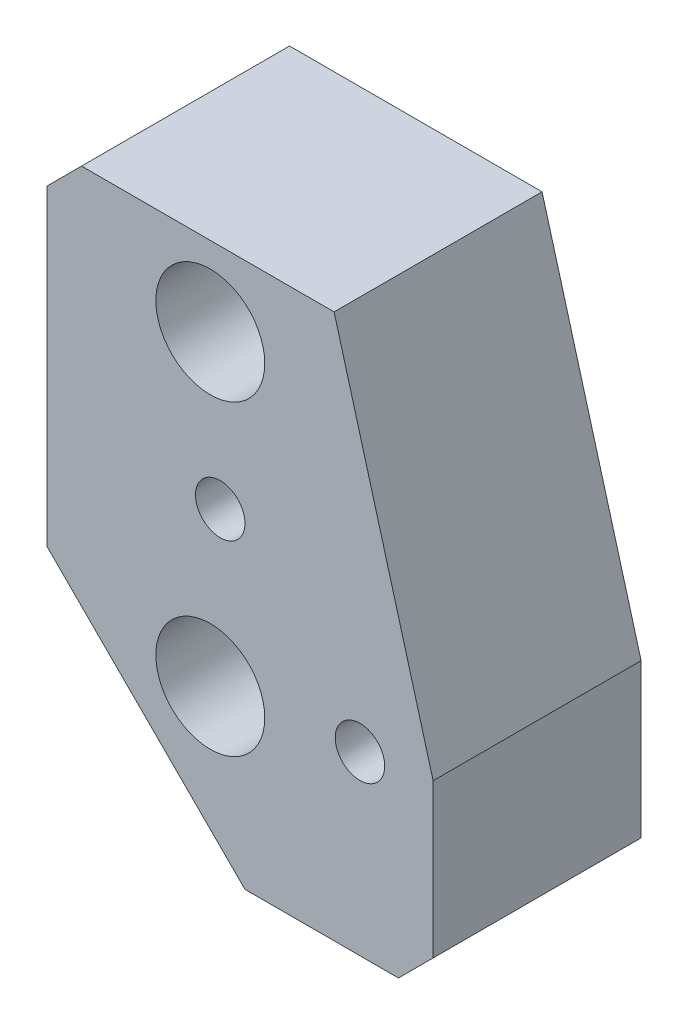
SolidWorks part; units mm, degrees
ref_plane "前视基准面" through (0, 0, 0) normal (0, 0, 1) x (1, 0, 0)
ref_plane "上视基准面" through (0, 0, 0) normal (0, 1, 0) x (1, 0, 0)
ref_plane "右视基准面" through (0, 0, 0) normal (1, 0, 0) x (0, 0, -1)
sketch "草图1" plane through (0, 0, 0) normal (0, 0, 1) x (1, 0, 0)
  line L0 (0, 20) -> (20, 0)
  line L1 (20, 0) -> (35.5, 0)
  line L2 (0, 20) -> (0, 51.5)
  line L3 (3.5, 55) -> (29, 55)
  line L4 (39, 3.5) -> (39, 19)
  line L5 (29, 55) -> (39, 19)
  line L6 (3.5, 55) -> (0, 51.5)
  line L7 (39, 3.5) -> (35.5, 0)
  dimension "D1" = 3.5
  dimension "D2" = 3.5
  dimension "D3" = 20
  dimension "D4" = 20
  dimension "D5" = 10
  dimension "D6" = 36
  dimension "D8" = 3.5
  dimension "D9" = 55
  dimension "D10" = 39
extrude "凸台-拉伸1" add sketch "草图1" along normal blind 21
sketch "草图2" plane through (0, 0, 21) normal (0, 0, 1) x (1, 0, 0)
  line L0 (0, 51.5) -> (0, 20) construction
  line L2 (29, 55) -> (3.5, 55) construction
  line L4 (20, 0) -> (35.5, 0) construction
  circle A0 centre (16.5, 47) radius 5.5
  circle A1 centre (16.5, 16) radius 5.5
  dimension "D1" = 11
  dimension "D2" = 11
  dimension "D3" = 16.5
  dimension "D4" = 8
  dimension "D5" = 16.5
  dimension "D6" = 16
extrude "切除-拉伸1" cut sketch "草图2" against normal blind 9
sketch "草图3" plane through (0, 0, 12) normal (0, 0, 1) x (1, 0, 0)
  circle A0 centre (16.5, 47) radius 3.5
  circle A1 centre (16.5, 16) radius 3.5
  dimension "D1" = 7
  dimension "D2" = 7
extrude "切除-拉伸2" cut sketch "草图3" against normal through all
hole_wizard "M6 螺纹孔1" positions "3D草图1" profile "草图4" tap size "M6" standard "GB"
sketch3d "3D草图1"
  line L0 (0, 51.5, 21) -> (0, 20, 21) construction
  line L1 (20, 0, 21) -> (35.5, 0, 21) construction
  line L2 (17.5, 32, 21) -> (34.0637, 15.3665, 21) construction
  point P0 (17.5, 32, 21)
  point P2 (31.6124, 17.8282, 21)
  dimension "D1" = 17.5
  dimension "D2" = 32
  dimension "D3" = 20
sketch "草图4" plane through (17.5, 32, 21) normal (1, 0, 0) x (0, -1, 0)
  line L0 (0, 0) -> (0, 18.5022)
  line L1 (0, 18.5022) -> (2.5, 17)
  line L2 (2.5, 17) -> (2.5, 0)
  line L5 (2.5, 0) -> (0, 0)
  line L10 (0, 18.5022) -> (-2.5, 17) construction
  line L11 (0, -6.35) -> (0, 107.95) construction
  dimension "螺纹孔钻头直径" = 5
  dimension "螺纹孔钻头深度" = 17
  dimension "导头角度" = 118
cosmetic thread "孔螺蚊线1" parameters "D1"=14, "D2"=6
cosmetic thread "孔螺蚊线2" parameters "D1"=14, "D2"=6
